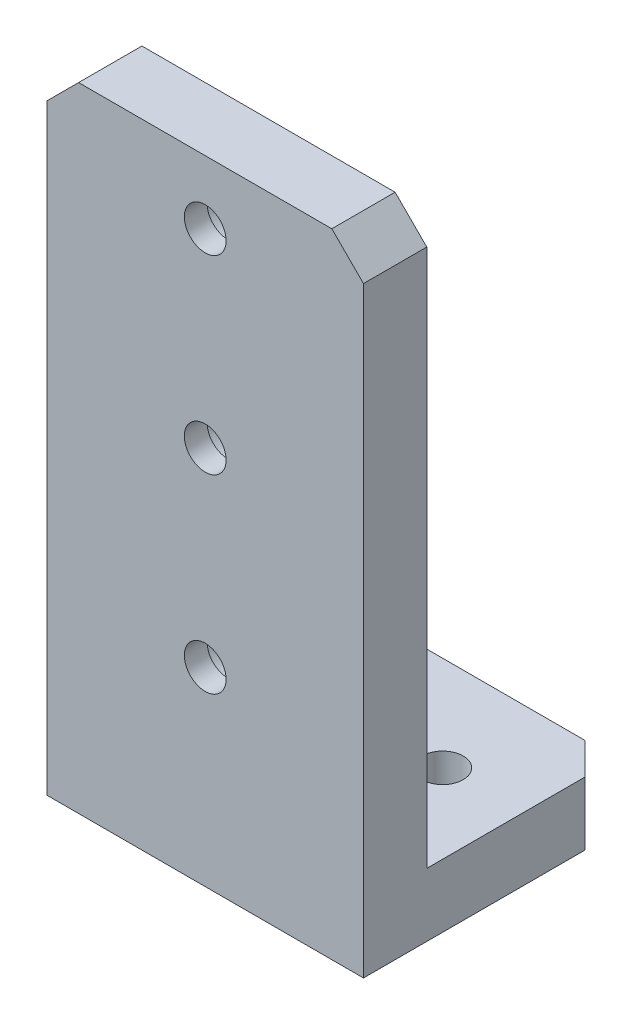
SolidWorks part; units mm, degrees
material "6061-T6"
ref_plane "前视基准面" through (0, 0, 0) normal (0, 0, 1) x (1, 0, 0)
ref_plane "上视基准面" through (0, 0, 0) normal (0, 1, 0) x (1, 0, 0)
ref_plane "右视基准面" through (0, 0, 0) normal (1, 0, 0) x (0, 0, -1)
sketch "草图2" plane through (0, 0, 0) normal (1, 0, 0) x (0, 0, -1)
  line L0 (0, 100) -> (0, 0)
  line L1 (0, 0) -> (40, 0)
  dimension "D1" = 40
  dimension "D2" = 100
extrude "拉伸-薄壁2" add sketch "草图2" along normal mid plane 50 thin thin type one direction reverse wall 10
hole_wizard "Ø6.5 (6.5) 直径孔1" positions "草图3" profile "草图4" hole size "Ø6.5" standard "ISO" end condition through all
sketch "草图3" plane through (0, 10, 0) normal (0, 1, 0) x (1, 0, 0)
  line L0 (0, 40) -> (0, 0) construction
  line L1 (25, 40) -> (-25, 40) construction
  point P0 (-12.5, 25)
  point P2 (12.5, 25)
  dimension "D1" = 15
  dimension "D2" = 25
sketch "草图4" plane through (-12.5, 10, -25) normal (1, 0, 0) x (0, 0, 1)
  line L0 (0, 0) -> (0, 10)
  line L1 (0, 10) -> (3.25, 10)
  line L2 (3.25, 10) -> (3.25, 0)
  line L5 (3.25, 0) -> (0, 0)
  line L11 (0, -6.35) -> (0, 107.95) construction
  dimension "通孔孔直径" = 6.5
  dimension "通孔孔深度" = 10
hole_wizard "M6 六角凹头螺钉的柱形沉头孔1" positions "草图5" profile "草图6" counterbore size "M6" standard "ISO" end condition through all
sketch "草图5" plane through (0, 0, -10) normal (0, 0, -1) x (-1, 0, 0)
  line L0 (0, 100) -> (0, 0) construction
  line L1 (-25, 100) -> (25, 100) construction
  line L3 (-25, 0) -> (25, 0) construction
  point P0 (0, 90)
  point P2 (0, 60)
  point P4 (0, 30)
  dimension "D1" = 30
  dimension "D2" = 30
  dimension "D3" = 30
sketch "草图6" plane through (0, 90, -10) normal (1, 0, 0) x (0, 1, 0)
  line L0 (0, 0) -> (0, 10)
  line L1 (0, 10) -> (3.3, 10)
  line L3 (3.3, 10) -> (3.3, 6.4)
  line L4 (3.3, 6.4) -> (5.5, 6.4)
  line L5 (5.5, 6.4) -> (5.5, 0)
  line L7 (5.5, 0) -> (0, 0)
  line L11 (0, -6.35) -> (0, 107.95) construction
  dimension "通孔孔直径" = 6.6
  dimension "通孔孔深度" = 10
  dimension "柱形沉头孔直径" = 11
  dimension "柱形沉头孔深度" = 6.4
chamfer "倒角1" distance 5 angle 45 4 edges at (-25, 5, -40) (25, 5, -40) (-25, 100, -5) (25, 100, -5)
